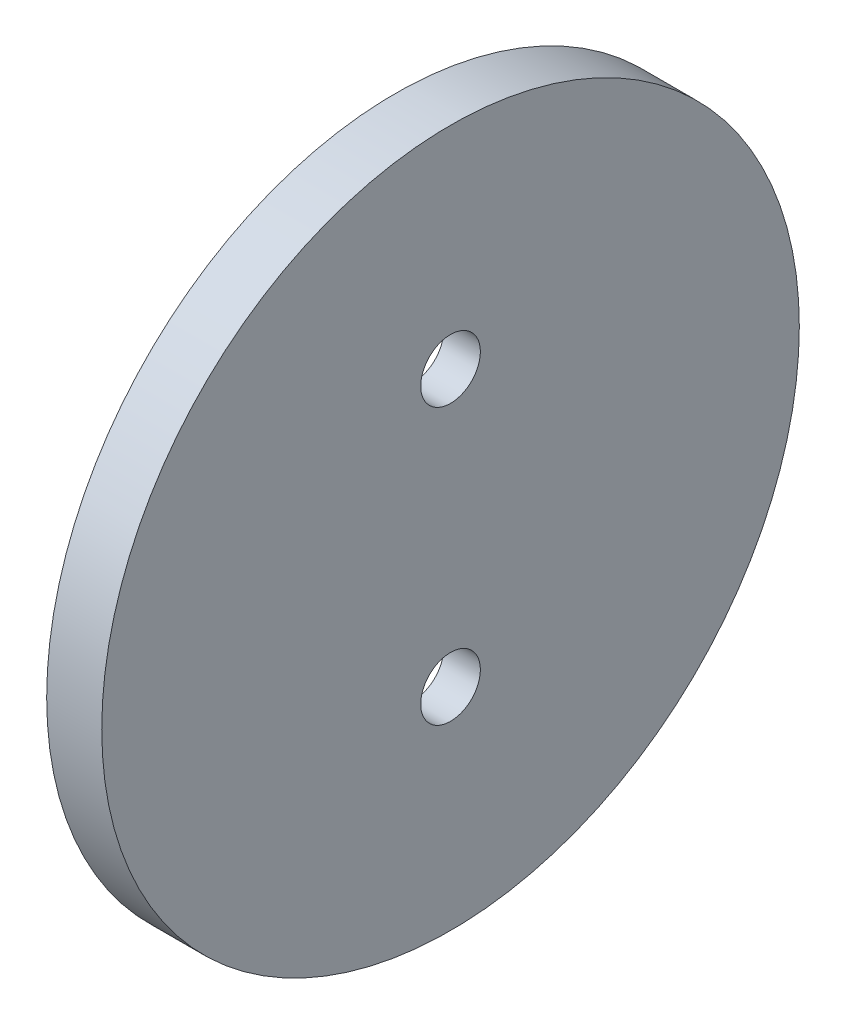
SolidWorks part; units mm, degrees
material "普通碳钢"
ref_plane "Front Plane" through (0, 0, 0) normal (0, 0, 1) x (1, 0, 0)
ref_plane "Top Plane" through (0, 0, 0) normal (0, 1, 0) x (1, 0, 0)
ref_plane "Right Plane" through (0, 0, 0) normal (1, 0, 0) x (0, 0, -1)
sketch "Sketch1" plane through (0, 0, 0) normal (0, 0, 1) x (1, 0, 0)
  line L0 (0, 0) -> (0, 38)
  line L1 (0, 38) -> (-6, 38)
  line L2 (-6, 38) -> (-6, 33)
  line L3 (-6, 33) -> (-4, 33)
  line L4 (-4, 33) -> (-4, 0)
  line L5 (-4, 0) -> (0, 0)
  line L6 (0, 0) -> (-42.5516, 0) construction
  dimension "D1" = 6
  dimension "D2" = 2
  dimension "D3" = 38
  dimension "D4" = 5
revolve "Revolve1" add sketch "Sketch1" angle 360 about L6
sketch "Sketch2" plane through (0, 0, 0) normal (1, 0, 0) x (0, 0, -1)
  line L0 (0, 46.573) -> (0, -49.3853) construction
  circle A0 centre (0, 15) radius 3.25
  circle A1 centre (0, -15) radius 3.25
  dimension "D1" = 6.5
  dimension "D2" = 6.5
  dimension "D3" = 15
  dimension "D4" = 15
extrude "Cut-Extrude1" cut sketch "Sketch2" against normal through all
